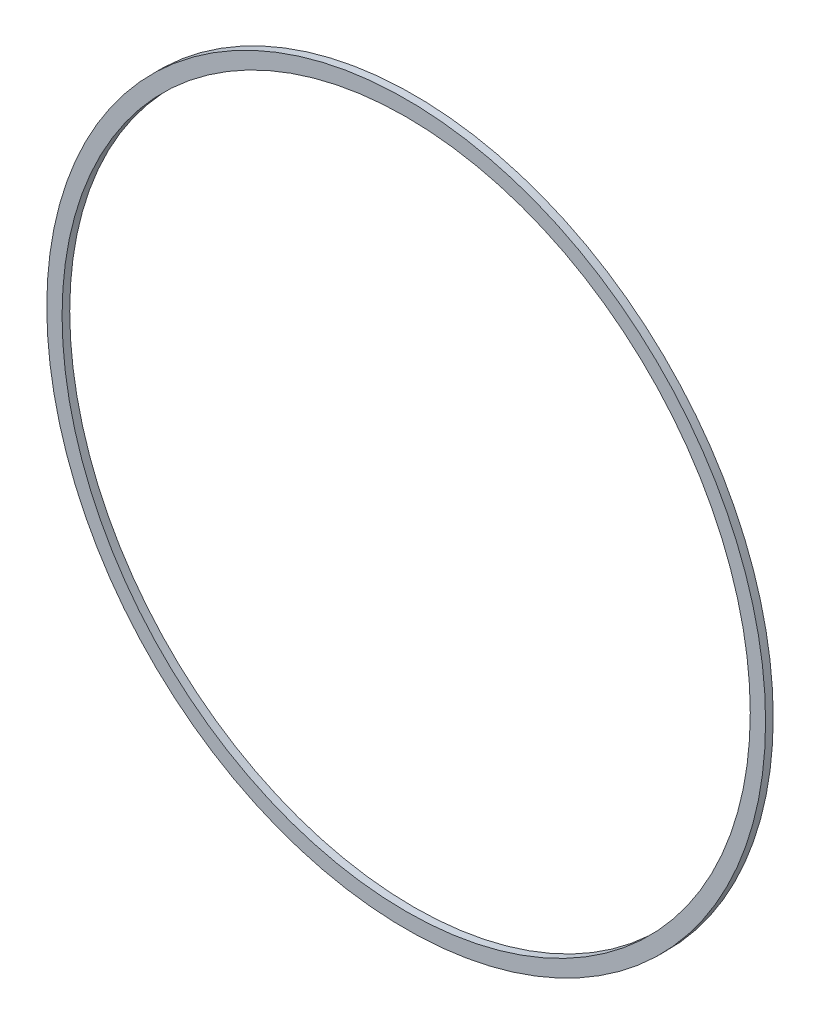
SolidWorks part; units mm, degrees
ref_plane "前视基准面" through (0, 0, 0) normal (0, 0, 1) x (1, 0, 0)
ref_plane "上视基准面" through (0, 0, 0) normal (0, 1, 0) x (1, 0, 0)
ref_plane "右视基准面" through (0, 0, 0) normal (1, 0, 0) x (0, 0, -1)
other "Configuration Table"
sketch "草图1" plane through (0, 0, 0) normal (0, 0, 1) x (1, 0, 0)
  circle A0 centre (0, 0) radius 94
  circle A1 centre (0, 0) radius 90
  point P0 (0, 0)
  dimension "D1" = 180
  dimension "D2" = 188
extrude "凸台-拉伸1" add sketch "草图1" against normal mid plane 2
